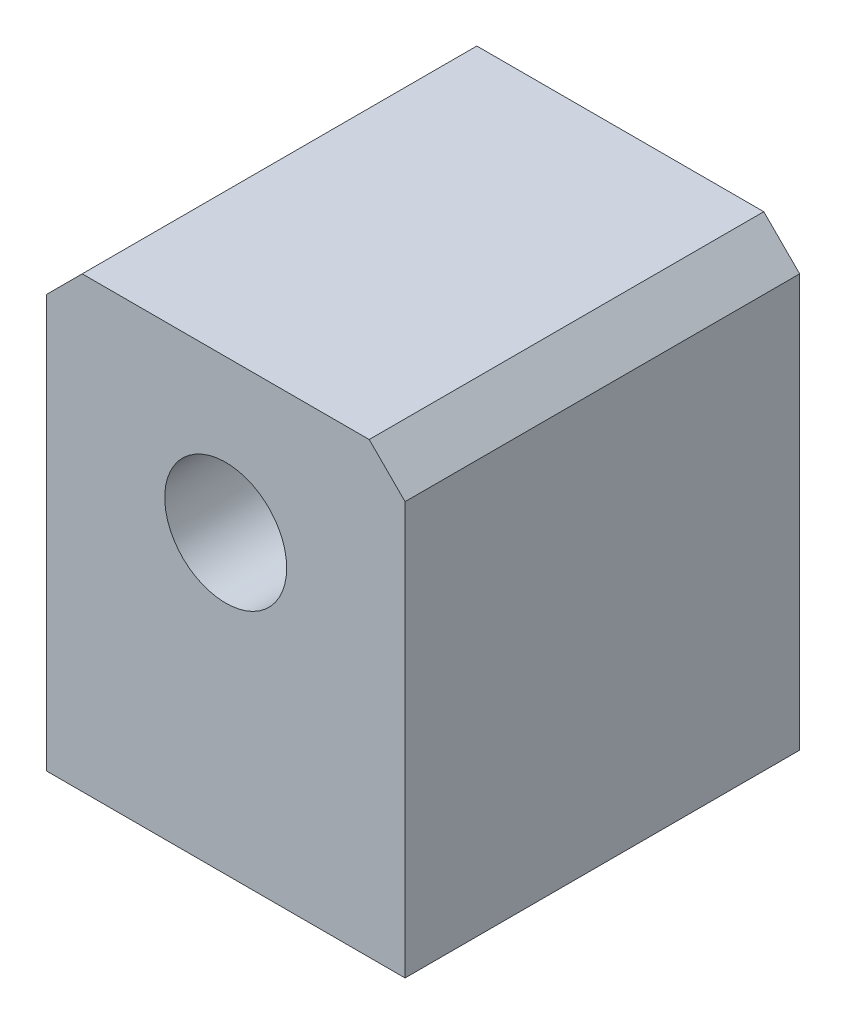
SolidWorks part; units mm, degrees
ref_plane "Front" through (0, 0, 0) normal (0, 0, 1) x (1, 0, 0)
ref_plane "Top" through (0, 0, 0) normal (0, 1, 0) x (1, 0, 0)
ref_plane "Right" through (0, 0, 0) normal (1, 0, 0) x (0, 0, -1)
sketch "Sketch1" plane through (0, 0, 0) normal (0, 0, 1) x (1, 0, 0)
  line L1 (-10, 12.5) -> (10, 12.5)
  line L2 (-10, 12.5) -> (-10, -12.5)
  line L3 (-10, -12.5) -> (10, -12.5)
  line L4 (10, 12.5) -> (10, -12.5)
  line L5 (-10, 12.5) -> (10, -12.5) construction
  line L6 (-10, -12.5) -> (10, 12.5) construction
  point P0 (0, 0)
  dimension "D1" = 20
  dimension "D2" = 25
extrude "Boss-Extrude1" add sketch "Sketch1" along normal mid plane 22
chamfer "Chamfer1" distance 2 angle 45 2 edges at (10, 12.5, 0) (-10, 12.5, 0)
hole_wizard "M8 Tapped Hole1" positions "Sketch3" profile "Sketch2" tap size "M8" standard "Gb" end condition through all
sketch "Sketch3" plane through (0, 0, 11) normal (0, 0, 1) x (1, 0, 0)
  line L0 (-10, -12.5) -> (10, -12.5) construction
  point P0 (0, 4)
  dimension "D1" = 16.5
sketch "Sketch2" plane through (0, 4, 11) normal (1, 0, 0) x (0, -1, 0)
  line L0 (0, 0) -> (0, 22)
  line L1 (0, 22) -> (3.4, 22)
  line L2 (3.4, 22) -> (3.4, 0)
  line L5 (3.4, 0) -> (0, 0)
  line L11 (0, -6.35) -> (0, 107.95) construction
  dimension "通孔螺纹孔钻头直径" = 6.8
  dimension "通孔螺纹孔钻头深度" = 22
cosmetic thread "Cosmetic thread 1" parameters "D2"=8
hole_wizard "M4 Tapped Hole1" positions "Sketch5" profile "Sketch4" tap size "M4" standard "Gb"
sketch "Sketch5" plane through (0, -12.5, 0) normal (0, -1, 0) x (-1, 0, 0)
  line L0 (10, -11) -> (10, 11) construction
  line L1 (10, -11) -> (-10, -11) construction
  line L2 (-10, -11) -> (-10, 11) construction
  line L3 (10, 11) -> (-10, 11) construction
  point P0 (6, -7)
  point P2 (-6, 7)
  dimension "D1" = 4
  dimension "D2" = 4
  dimension "D3" = 4
  dimension "D4" = 4
sketch "Sketch4" plane through (-6, -12.5, 7) normal (1, 0, 0) x (0, 0, -1)
  line L0 (0, 0) -> (0, 12.4914)
  line L1 (0, 12.4914) -> (1.65, 11.5)
  line L2 (1.65, 11.5) -> (1.65, 0)
  line L5 (1.65, 0) -> (0, 0)
  line L10 (0, 12.4914) -> (-1.65, 11.5) construction
  line L11 (0, -6.35) -> (0, 107.95) construction
  dimension "螺纹孔钻头直径" = 3.3
  dimension "螺纹孔钻头深度" = 11.5
  dimension "导头角度" = 118
cosmetic thread "Cosmetic thread 2"
cosmetic thread "Cosmetic thread 3"
hole_wizard "Ø4.0 (4) Diameter Hole1" positions "Sketch7" profile "Sketch6" hole size "Ø4.0" standard "Gb"
sketch "Sketch7" plane through (0, -12.5, 0) normal (0, -1, 0) x (-1, 0, 0)
  line L0 (10, 11) -> (-10, 11) construction
  line L1 (10, -11) -> (10, 11) construction
  line L2 (10, -11) -> (-10, -11) construction
  line L3 (-10, -11) -> (-10, 11) construction
  point P0 (-6, -7)
  point P2 (6, 7)
  dimension "D1" = 4
  dimension "D2" = 4
  dimension "D3" = 4
  dimension "D4" = 4
sketch "Sketch6" plane through (6, -12.5, 7) normal (1, 0, 0) x (0, 0, -1)
  line L0 (0, 0) -> (0, 9.2017)
  line L1 (0, 9.2017) -> (2, 8)
  line L2 (2, 8) -> (2, 0)
  line L5 (2, 0) -> (0, 0)
  line L10 (0, 9.2017) -> (-2, 8) construction
  line L11 (0, -6.35) -> (0, 107.95) construction
  dimension "孔直径" = 4
  dimension "孔深度" = 8
  dimension "导头角度" = 118
